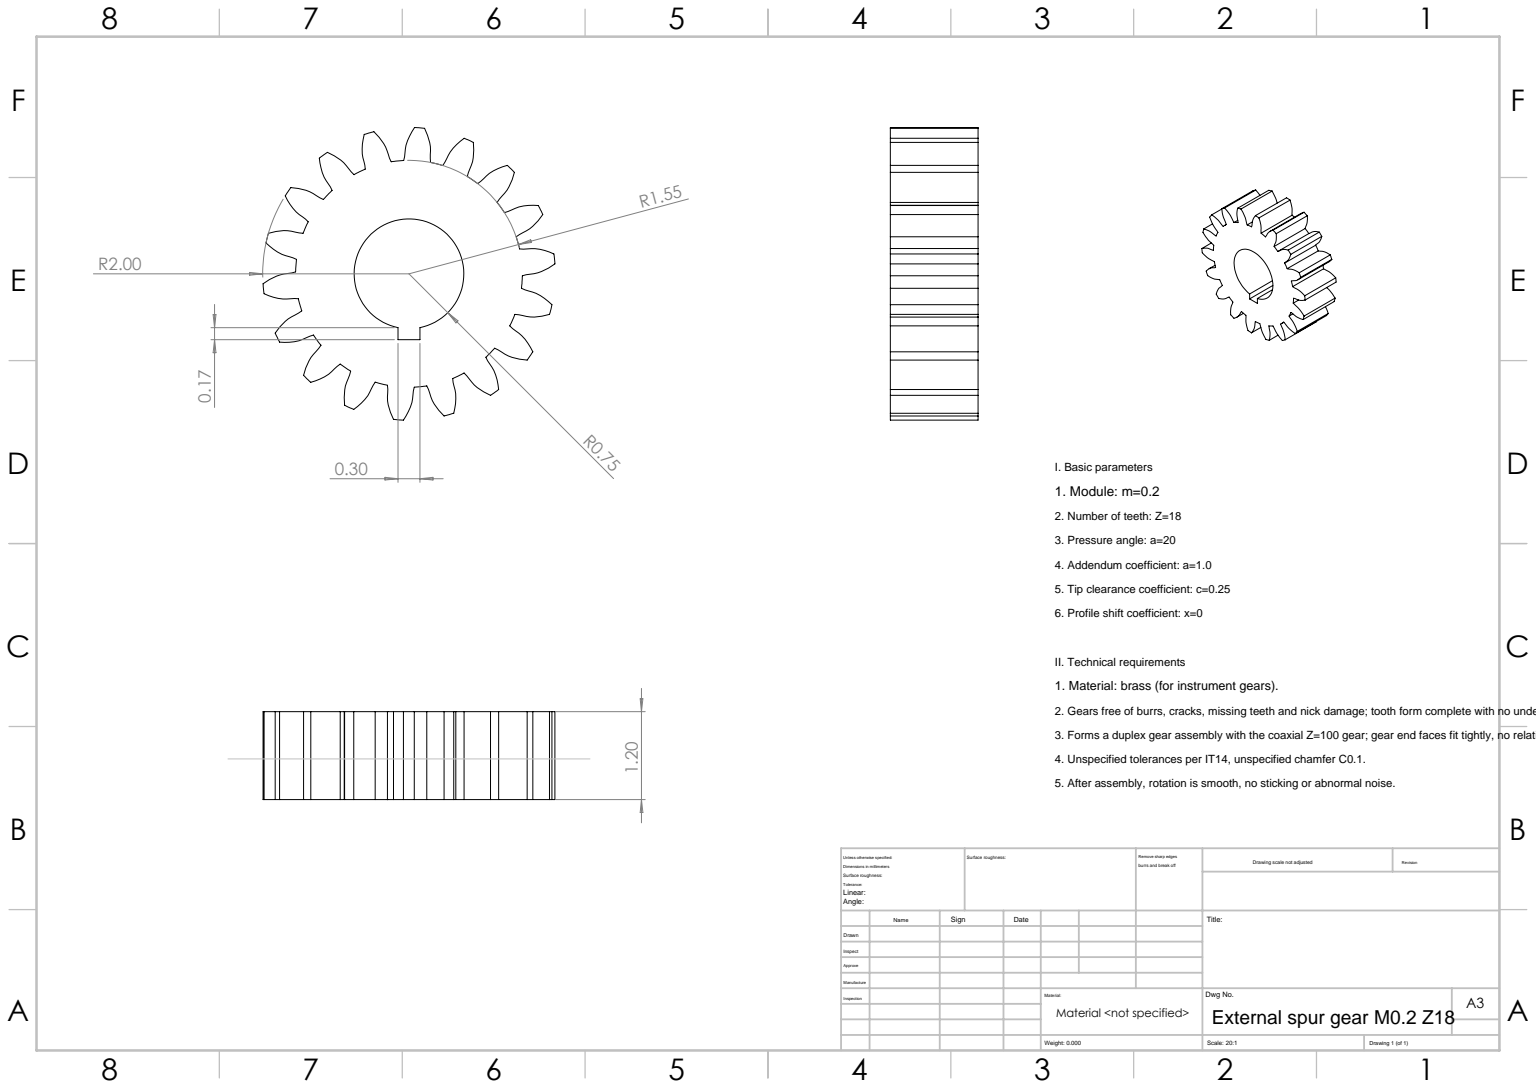
from build123d import *

# Parameters (mm, degrees)
SKETCH1_R           = 1.55
SKETCH1_R_2         = 0.75
BOSS_EXTRUDE1_DEPTH = 1.2
BOSS_EXTRUDE2_DEPTH = 1.2
CIRPATTERN1_COUNT   = 18
SKETCH3_W           = 0.3
SKETCH3_H           = 0.3
CUT_EXTRUDE1_DEPTH  = 10


with BuildPart() as part:
    # Sketch1 → Boss-Extrude1 (new body)
    with BuildSketch(Plane.XY):
        Circle(SKETCH1_R)
        Circle(SKETCH1_R_2, mode=Mode.SUBTRACT)
    extrude(amount=BOSS_EXTRUDE1_DEPTH)

    # Sketch2 → Boss-Extrude2 (add)
    with BuildSketch(Plane.XY):
        with BuildLine():
            ThreePointArc((1.981463542, 0.271665661), (1.989570196, 0.203986362), (1.995365862, 0.136070122))
            add(Edge.make_bspline(
                [(1.995365862, 0.136070122), (1.957290835, 0.10836634), (1.898409877, 0.070688485), (1.815670495, 0.032135256), (1.709099147, -0.00717099), (1.61481981, -0.002339743), (1.549781348, -0.0260341)],
                knots=[0, 0, 0, 0, 0.294268927, 0.434360997, 0.569740734, 1, 1, 1, 1], degree=3))
            ThreePointArc((1.549781348, -0.0260341), (1.541916902, 0.158089431), (1.512254902, 0.339978105))
            add(Edge.make_bspline(
                [(1.981463542, 0.271665661), (1.938558951, 0.291066777), (1.873257336, 0.316012459), (1.784416044, 0.33697389), (1.67208581, 0.353836627), (1.580748345, 0.329974487), (1.512254902, 0.339978105)],
                knots=[0, 0, 0, 0, 0.294268927, 0.434360997, 0.569740734, 1, 1, 1, 1], degree=3))
        make_face()
    boss_extrude2 = extrude(amount=BOSS_EXTRUDE2_DEPTH)

    # CirPattern1: Boss-Extrude2 ×18 about axis
    cirpattern1_axis = Axis((0, 0, 1.2), (0, 0, -1))
    for i in range(1, CIRPATTERN1_COUNT):
        add(boss_extrude2.rotate(cirpattern1_axis, i * 360 / CIRPATTERN1_COUNT))

    # Sketch3 → Cut-Extrude1 (cut)
    with BuildSketch(Plane.XY.offset(1.2)):
        with Locations((0, -0.75)):
            Rectangle(SKETCH3_W, SKETCH3_H)
    extrude(amount=-CUT_EXTRUDE1_DEPTH, mode=Mode.SUBTRACT)


solid = part.part
